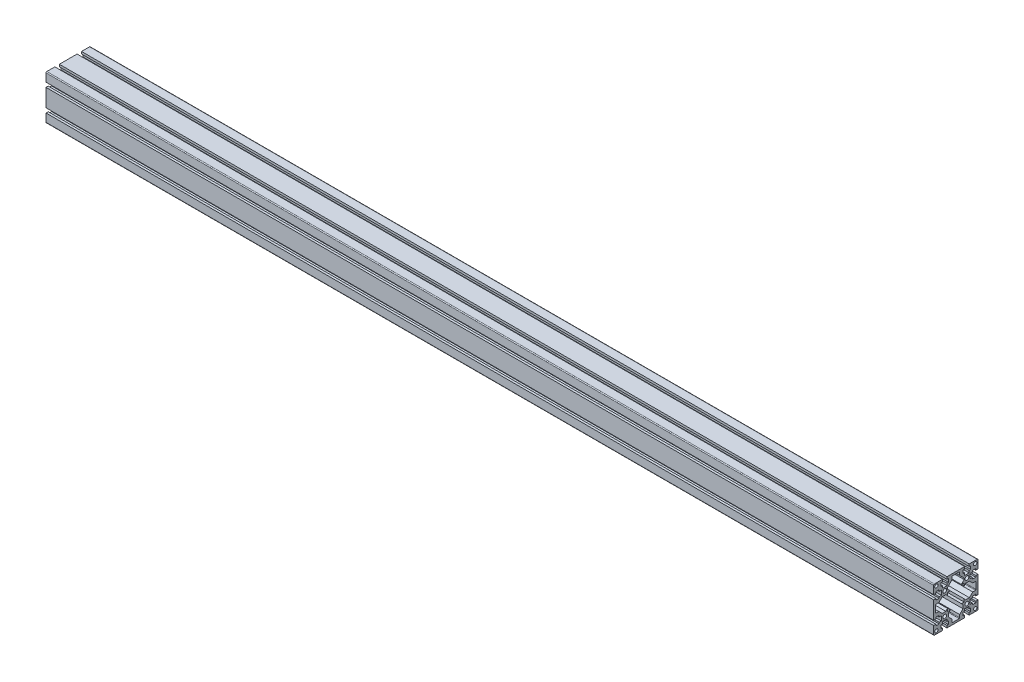
SolidWorks part; units mm, degrees
ref_plane "Front Plane" through (0, 0, 0) normal (0, 0, 1) x (1, 0, 0)
ref_plane "Top Plane" through (0, 0, 0) normal (0, 1, 0) x (1, 0, 0)
ref_plane "Right Plane" through (0, 0, 0) normal (1, 0, 0) x (0, 0, -1)
sketch "草图1" plane through (0, 0, 0) normal (0, 0, 1) x (1, 0, 0)
  line L0 (-530.3448, 0) -> (1069.6552, 0)
  dimension "D1" = 1600
other "Aluminium profile 80 X 80G X R1.5(1)"
ref_plane "Plane2" through (-530.3448, 0, 0) normal (1, 0, 0) x (0, 1, 0)
sketch "Sketch1" plane through (-530.3448, 0, 0) normal (1, 0, 0) x (0, 1, 0)
  line L0 (0, 40) -> (0, 0) construction
  line L1 (0, 0) -> (40, 0) construction
  line L2 (-24.05, 40) -> (-24.05, 36)
  line L3 (-38.5, 40) -> (-24.05, 40)
  line L4 (-40, 38.5) -> (-40, 24.05)
  line L5 (-38.5, -40) -> (-24.05, -40)
  line L6 (40, 38.5) -> (40, 24.05)
  line L7 (-24.05, 36) -> (-26.75, 36)
  line L8 (-26.75, 36) -> (-26.75, 30)
  line L9 (-26.75, 30) -> (-24.05, 30)
  line L10 (-24.05, 30) -> (-24.05, 26)
  line L11 (-24.05, 26) -> (-15.95, 26)
  line L12 (-15.95, 26) -> (-15.95, 30)
  line L13 (-15.95, 30) -> (-13.25, 30)
  line L14 (-13.25, 30) -> (-13.25, 36)
  line L15 (-13.25, 36) -> (-15.95, 36)
  line L16 (-15.95, 36) -> (-15.95, 40)
  line L17 (-40, 15.95) -> (-36, 15.95)
  line L18 (-36, 15.95) -> (-36, 13.25)
  line L19 (-15.95, 40) -> (15.95, 40)
  line L20 (-20, 20) -> (-20, 40) construction
  line L21 (20, 20) -> (20, 40) construction
  line L22 (15.95, 36) -> (15.95, 40)
  line L23 (13.25, 36) -> (15.95, 36)
  line L24 (13.25, 30) -> (13.25, 36)
  line L25 (15.95, 30) -> (13.25, 30)
  line L26 (-36, 13.25) -> (-30, 13.25)
  line L27 (-30, 13.25) -> (-30, 15.95)
  line L28 (-26, 15.95) -> (-26, 24.05)
  line L29 (-26, 24.05) -> (-30, 24.05)
  line L30 (-30, 24.05) -> (-30, 26.75)
  line L31 (-30, 26.75) -> (-36, 26.75)
  line L32 (-36, 26.75) -> (-36, 24.05)
  line L33 (-36, 24.05) -> (-40, 24.05)
  line L34 (-30, 15.95) -> (-26, 15.95)
  line L35 (15.95, 26) -> (15.95, 30)
  line L36 (24.05, 26) -> (15.95, 26)
  line L37 (24.05, 30) -> (24.05, 26)
  line L38 (26.75, 30) -> (24.05, 30)
  line L39 (26.75, 36) -> (26.75, 30)
  line L40 (24.05, 36) -> (26.75, 36)
  line L41 (24.05, 40) -> (24.05, 36)
  line L42 (24.05, -40) -> (24.05, -36)
  line L43 (24.05, -36) -> (26.75, -36)
  line L44 (26.75, -36) -> (26.75, -30)
  line L45 (26.75, -30) -> (24.05, -30)
  line L46 (24.05, -30) -> (24.05, -26)
  line L47 (24.05, -26) -> (15.95, -26)
  line L48 (15.95, -26) -> (15.95, -30)
  line L49 (15.95, -30) -> (13.25, -30)
  line L50 (13.25, -30) -> (13.25, -36)
  line L51 (13.25, -36) -> (15.95, -36)
  line L52 (15.95, -36) -> (15.95, -40)
  line L53 (-15.95, -36) -> (-15.95, -40)
  line L54 (-13.25, -36) -> (-15.95, -36)
  line L55 (-13.25, -30) -> (-13.25, -36)
  line L56 (-15.95, -30) -> (-13.25, -30)
  line L57 (-15.95, -26) -> (-15.95, -30)
  line L58 (-24.05, -26) -> (-15.95, -26)
  line L59 (-24.05, -30) -> (-24.05, -26)
  line L60 (-26.75, -30) -> (-24.05, -30)
  line L61 (-26.75, -36) -> (-26.75, -30)
  line L62 (-24.05, -36) -> (-26.75, -36)
  line L63 (-24.05, -40) -> (-24.05, -36)
  line L64 (-30, -15.95) -> (-26, -15.95)
  line L65 (-36, -26.75) -> (-36, -24.05)
  line L66 (-30, -26.75) -> (-36, -26.75)
  line L67 (-30, -24.05) -> (-30, -26.75)
  line L68 (-26, -24.05) -> (-30, -24.05)
  line L69 (-26, -15.95) -> (-26, -24.05)
  line L70 (-30, -13.25) -> (-30, -15.95)
  line L71 (-36, -13.25) -> (-30, -13.25)
  line L72 (-36, -15.95) -> (-36, -13.25)
  line L73 (36, 24.05) -> (40, 24.05)
  line L74 (40, 15.95) -> (36, 15.95)
  line L75 (36, -15.95) -> (36, -13.25)
  line L76 (36, -13.25) -> (30, -13.25)
  line L77 (30, -13.25) -> (30, -15.95)
  line L78 (26, -15.95) -> (26, -24.05)
  line L79 (26, -24.05) -> (30, -24.05)
  line L80 (30, -24.05) -> (30, -26.75)
  line L81 (30, -26.75) -> (36, -26.75)
  line L82 (36, -26.75) -> (36, -24.05)
  line L83 (30, -15.95) -> (26, -15.95)
  line L84 (30, 15.95) -> (26, 15.95)
  line L85 (36, 26.75) -> (36, 24.05)
  line L86 (30, 26.75) -> (36, 26.75)
  line L87 (30, 24.05) -> (30, 26.75)
  line L88 (26, 24.05) -> (30, 24.05)
  line L89 (26, 15.95) -> (26, 24.05)
  line L90 (30, 13.25) -> (30, 15.95)
  line L91 (36, 13.25) -> (30, 13.25)
  line L92 (36, 15.95) -> (36, 13.25)
  line L93 (-36, -15.95) -> (-40, -15.95)
  line L94 (-36, -24.05) -> (-40, -24.05)
  line L95 (36, -15.95) -> (40, -15.95)
  line L96 (36, -24.05) -> (40, -24.05)
  line L97 (-13, 18) -> (-10, 15)
  line L98 (-15, 15) -> (-10, 15)
  line L99 (-15, 15) -> (-15, 10)
  line L100 (-15, -15) -> (-10, -15)
  line L101 (15, 15) -> (15, 10)
  line L102 (-18, 13) -> (-15, 10)
  line L104 (13, 18) -> (10, 15)
  line L105 (13, -18) -> (10, -15)
  line L106 (20, -15) -> (15, -10)
  line L107 (-18, -13) -> (-15, -10)
  line L108 (-13, -18) -> (-10, -15)
  line L109 (15, -10) -> (15, -15)
  line L110 (10, 15) -> (15, 15)
  line L111 (-15, -10) -> (-15, -15)
  line L112 (10, -15) -> (15, -15)
  line L113 (15, 10) -> (20, 15)
  line L235 (24.05, 40) -> (38.5, 40)
  line L249 (-40, 15.95) -> (-40, -15.95)
  line L250 (-20, 20) -> (-26, 20) construction
  line L264 (40, 15.95) -> (40, -15.95)
  line L265 (-13, 24.5) -> (-7, 30.5)
  line L266 (-7, 30.5) -> (-7, 35.5)
  line L267 (7, 35.5) -> (7, 30.5)
  line L268 (7, 30.5) -> (13, 24.5)
  line L269 (-6, -36.5) -> (6, -36.5)
  line L270 (-13, 24.5) -> (-13, 18)
  line L271 (-35.5, 7) -> (-30.5, 7)
  line L272 (-30.5, 7) -> (-24.5, 13)
  line L273 (-24.5, 13) -> (-18, 13)
  line L274 (13, 24.5) -> (13, 18)
  line L275 (-15.95, -40) -> (15.95, -40)
  line L276 (35.5, 7) -> (30.5, 7)
  line L277 (30.5, 7) -> (22.5, 15)
  line L278 (24.05, -40) -> (38.5, -40)
  line L279 (20, 15) -> (22.5, 15)
  line L333 (-13, -24.5) -> (-13, -18)
  line L336 (-13, -24.5) -> (-7, -30.5)
  line L385 (-7, -30.5) -> (-7, -35.5)
  line L386 (-36.5, 6) -> (-36.5, -6)
  line L387 (7, -35.5) -> (7, -30.5)
  line L429 (7, -30.5) -> (13, -24.5)
  line L430 (13, -24.5) -> (13, -18)
  line L494 (20, -15) -> (22.5, -15)
  line L496 (30.5, -7) -> (22.5, -15)
  line L497 (35.5, -7) -> (30.5, -7)
  line L498 (-24.5, -13) -> (-18, -13)
  line L499 (-30.5, -7) -> (-24.5, -13)
  line L500 (-35.5, -7) -> (-30.5, -7)
  line L512 (40, -24.05) -> (40, -38.5)
  line L519 (-40, -24.05) -> (-40, -38.5)
  line L520 (-6, 36.5) -> (6, 36.5)
  line L523 (36.5, 6) -> (36.5, -6)
  circle A0 centre (-20, 20) radius 3.4
  circle A2 centre (20, 20) radius 3.4
  circle A3 centre (20, -20) radius 3.4
  circle A7 centre (-20, -20) radius 3.4
  arc A8 (-38.5, 40) -> (-40, 38.5) centre (-38.5, 38.5) ccw
  arc A9 (-40, -38.5) -> (-38.5, -40) centre (-38.5, -38.5) ccw
  arc A10 (38.5, -40) -> (40, -38.5) centre (38.5, -38.5) ccw
  arc A11 (38.5, 40) -> (40, 38.5) centre (38.5, 38.5) cw
  circle A12 centre (-35, 35) radius 3
  circle A13 centre (35, 35) radius 3
  circle A14 centre (35, -35) radius 3
  arc A15 (-6, 36.5) -> (-7, 35.5) centre (-6, 35.5) ccw
  arc A16 (6, 36.5) -> (7, 35.5) centre (6, 35.5) cw
  arc A17 (-36.5, 6) -> (-35.5, 7) centre (-35.5, 6) cw
  arc A18 (-36.5, -6) -> (-35.5, -7) centre (-35.5, -6) ccw
  arc A19 (36.5, -6) -> (35.5, -7) centre (35.5, -6) cw
  arc A20 (36.5, 6) -> (35.5, 7) centre (35.5, 6) ccw
  arc A21 (6, -36.5) -> (7, -35.5) centre (6, -35.5) ccw
  arc A22 (-6, -36.5) -> (-7, -35.5) centre (-6, -35.5) cw
  point P48 (-20, 20)
  point P97 (0, 0)
  point P104 (-7, 36.5)
  point P185 (40, 40)
  point P187 (40, -40)
  point P188 (-40, -40)
  point P190 (-40, 40)
  dimension "D1" = 80
  dimension "D2" = 80
  dimension "D3" = 20
  dimension "D4" = 8.1
  dimension "D5" = 45
  dimension "D6" = 7
  dimension "D7" = 13.5
  dimension "D8" = 6
  dimension "D12" = 5
  dimension "D13" = 5
  dimension "D14" = 20
  dimension "D18" = 1
  dimension "D19" = 14
  dimension "D15" = 6.8
  dimension "D27" = 45
  dimension "D20" = 1.5
  dimension "D11" = 6
  dimension "D9" = 4
  dimension "D10" = 14
  dimension "D16" = 14
  dimension "D17" = 45
  dimension "D21" = 3.5
  dimension "D22" = 3.5
  dimension "D23" = 73
  dimension "D24" = 30
  dimension "D25" = 30
  dimension "D26" = 45
  dimension "D28" = 5
sketch "Sketch10" plane through (1069.6552, 0, 0) normal (1, 0, 0) x (0, 0, -1)
  circle A0 centre (35, -35) radius 3
  circle A1 centre (-35, -35) radius 3 construction
  circle A2 centre (35, 35) radius 3 construction
  dimension "D1" = 6
  dimension "D2" = 70
  dimension "D3" = 70
extrude "Cut-Extrude1" cut sketch "Sketch10" against normal through all
